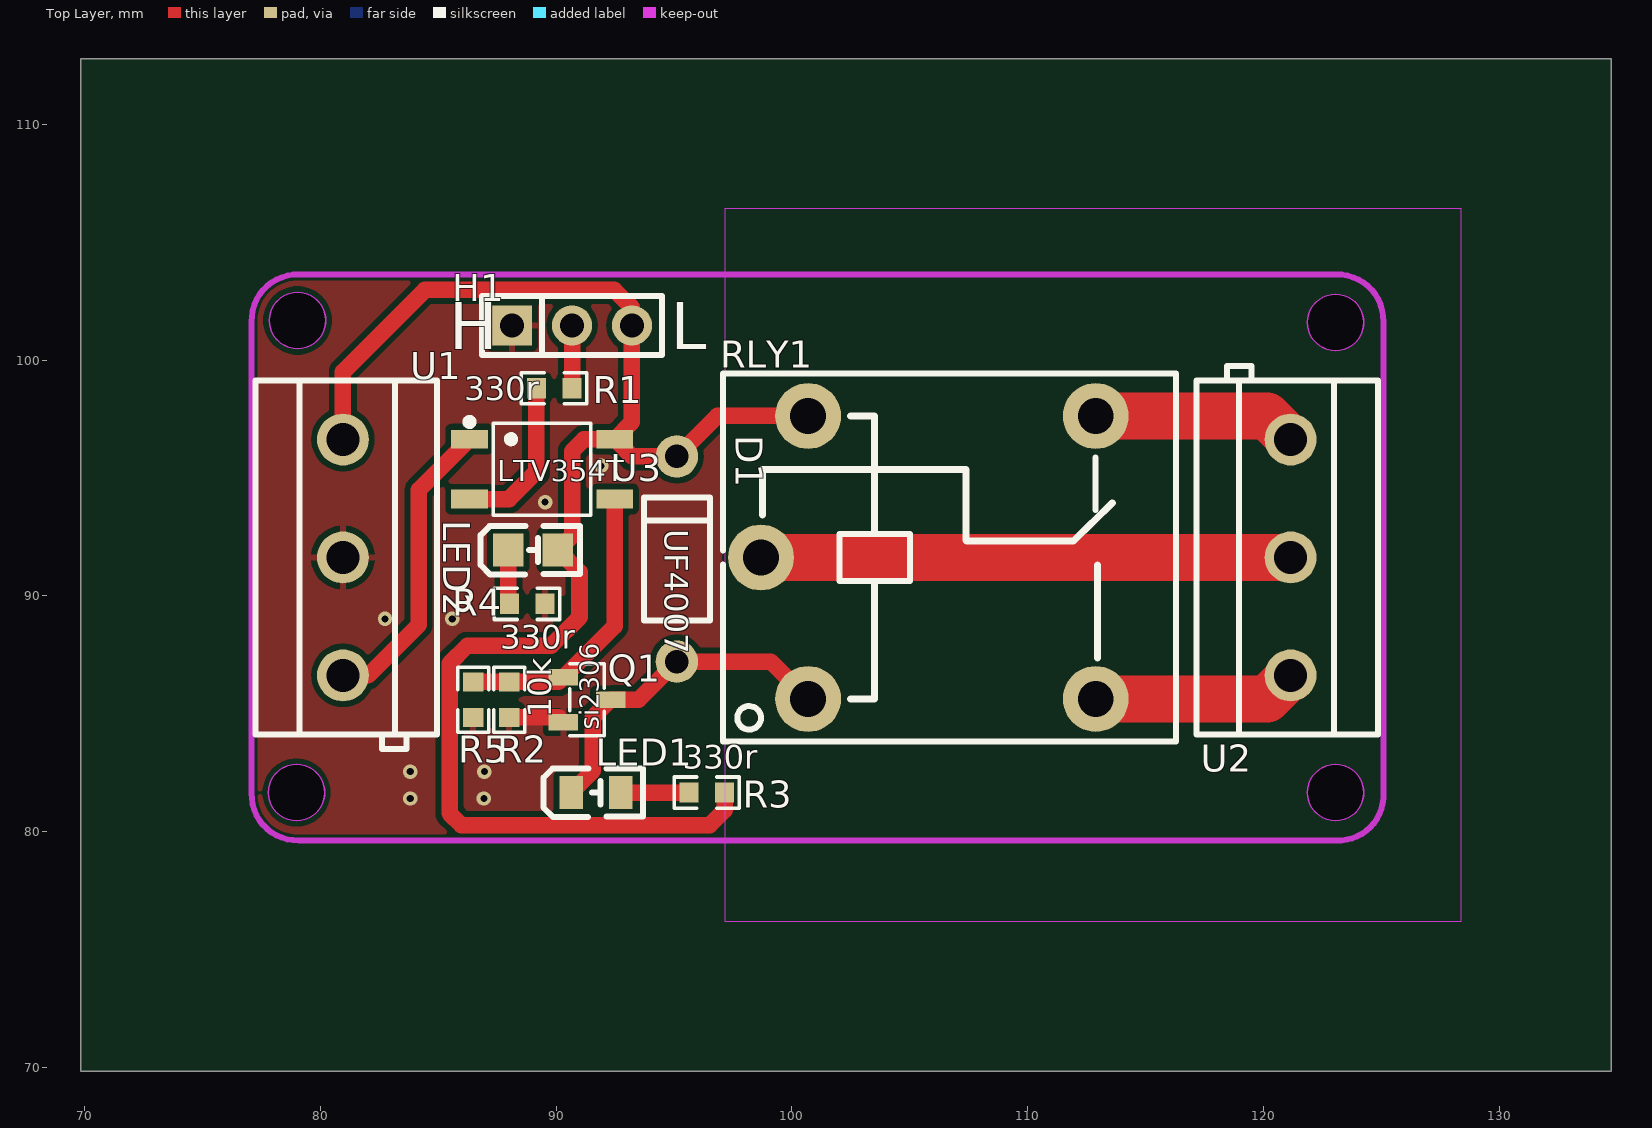
[diagram p0: Top Layer view]
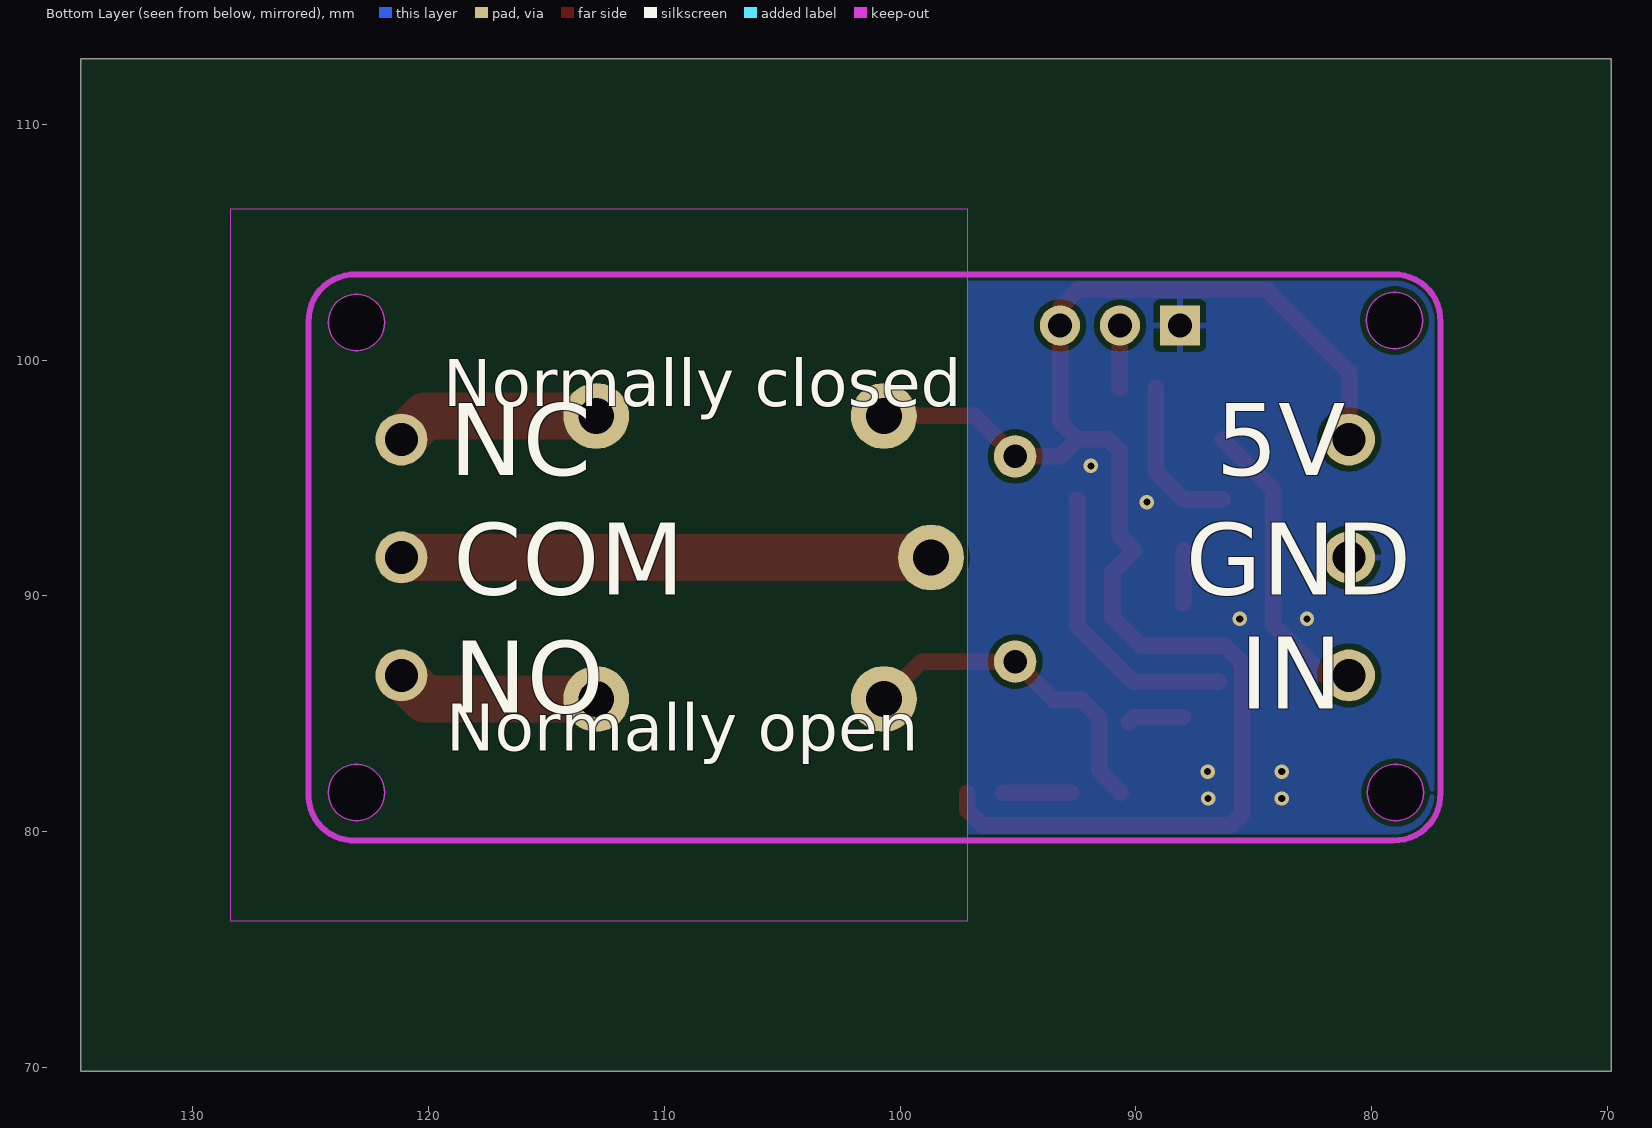
[diagram p1: Bottom Layer view, seen from below]
# Altium PCB MISC49931.pcbdoc
Units mm, origin at the board's own origin, x right, y up, seen from the top; angles counter-clockwise.
Board outline 64.9 x 42.93 mm, 2 copper layers (Top Layer, Bottom Layer), stack 1.58 mm thick; 14 components, 12 nets, 37 pads, 8 vias.

## Layer stack, top to bottom
Top Solder Mask Layer: solder mask 0.01, Dk 3.3
Top Layer: signal copper 0.035
Dielectric1: surface 1.51, FR4, Dk 4.5
Bottom Layer: signal copper 0.035
Bottom Solder Mask Layer: solder mask 0.01, Dk 3.3

## Board outline
134.747,69.85 69.85,69.85 69.85,112.776 134.747,112.776
cut-out: 80.233,101.684 cw(c79.037,101.684) 77.84,101.684 cw(c79.037,101.684)
cut-out: 80.191,81.661 cw(c78.994,81.661) 77.797,81.661 cw(c78.994,81.661)
cut-out: 124.26,81.661 cw(c123.063,81.661) 121.866,81.661 cw(c123.063,81.661)
cut-out: 124.26,101.6 cw(c123.063,101.6) 121.866,101.6 cw(c123.063,101.6)

## Design rules (kind name [scope] priority, off if disabled: settings)
BoardOutlineClearance copperThickness2oz_1 [All] p2 off: genericclearance=0.203 ignorepadtopadclearanceinfootprint=FALSE except(0: Arc-SplitContinuation Track-SplitContinuation SMDPad-SplitContinuation THPad-SplitContinuation Via-SplitContinuation Fill-SplitContinuation Region-SplitContinuation Poly-SplitContinuation Text-SplitContinuation Hole-SplitContinuation; 0.152: Arc-CutoutEdge SMDPad-CutoutEdge THPad-CutoutEdge Via-CutoutEdge Fill-CutoutEdge Region-CutoutEdge Text-CutoutEdge; 0.176: Hole-OutlineEdge Hole-CutoutEdge; 0.254: Poly-OutlineEdge Poly-CutoutEdge; 0.3: Arc-OutlineEdge Track-OutlineEdge SMDPad-OutlineEdge THPad-OutlineEdge Via-OutlineEdge Fill-OutlineEdge Region-OutlineEdge Text-OutlineEdge Track-CutoutEdge)
BoardOutlineClearance copperThickness1oz_1 [All] p4: genericclearance=0.102 ignorepadtopadclearanceinfootprint=FALSE except(0: Arc-SplitContinuation Track-SplitContinuation SMDPad-SplitContinuation THPad-SplitContinuation Via-SplitContinuation Fill-SplitContinuation Region-SplitContinuation Poly-SplitContinuation Text-SplitContinuation Hole-SplitContinuation; 0.152: SMDPad-CutoutEdge THPad-CutoutEdge Via-CutoutEdge Fill-CutoutEdge Region-CutoutEdge Text-CutoutEdge; 0.176: Hole-OutlineEdge Hole-CutoutEdge; 0.254: Poly-OutlineEdge Poly-CutoutEdge; 0.3: Arc-OutlineEdge Track-OutlineEdge SMDPad-OutlineEdge THPad-OutlineEdge Via-OutlineEdge Fill-OutlineEdge Region-OutlineEdge Text-OutlineEdge Arc-CutoutEdge Track-CutoutEdge)
Clearance copperThickness2oz [All] p1 off: gap=0.203 ignorepadtopadclearanceinfootprint=FALSE except(0.152: SMDPad-Track SMDPad-SMDPad THPad-Track SMDPad-THPad THPad-THPad Track-Via SMDPad-Via THPad-Via Via-Via Fill-Track Region-Track Fill-SMDPad Region-SMDPad Fill-THPad Region-THPad Fill-Via Region-Via Fill-Fill Fill-Region Region-Region Arc-Track Arc-SMDPad Arc-THPad Arc-Via Fill-Arc Region-Arc Arc-Arc Text-Track SMDPad-Text Text-THPad Text-Via Fill-Text Region-Text Arc-Text Text-Text; 0.176: Hole-Track Hole-SMDPad Hole-THPad Hole-Via Fill-Hole Region-Hole Hole-Arc Hole-Text; 0.254: Poly-Track Poly-SMDPad Poly-THPad Poly-Via Poly-Fill Poly-Region Poly-Poly Poly-Arc Poly-Text Poly-Hole)
Clearance copperThickness1oz [All] p3: gap=0.102 ignorepadtopadclearanceinfootprint=FALSE except(0.152: SMDPad-Track SMDPad-SMDPad THPad-Track SMDPad-THPad THPad-THPad Track-Via SMDPad-Via THPad-Via Via-Via Fill-Track Region-Track Fill-SMDPad Region-SMDPad Fill-THPad Region-THPad Fill-Via Region-Via Fill-Fill Fill-Region Region-Region Arc-Track Arc-SMDPad Arc-THPad Arc-Via Fill-Arc Region-Arc Arc-Arc Text-Track SMDPad-Text Text-THPad Text-Via Fill-Text Region-Text Arc-Text Text-Text; 0.176: Hole-Track Hole-SMDPad Hole-THPad Hole-Via Fill-Hole Region-Hole Hole-Arc Hole-Text; 0.254: Poly-Track Poly-SMDPad Poly-THPad Poly-Via Poly-Fill Poly-Region Poly-Poly Poly-Arc Poly-Text Poly-Hole)
DiffPairsRouting differentialPair [All] p1: maxlimit=0.152 minlimit=0.152 mostfreqgap=0.152 toplayer_minwidth=0.127 toplayer_prefwidth=0.254 toplayer_maxwidth=2.54 toplayer_mingap=0.152 toplayer_prefgap=0.152 toplayer_maxgap=0.152 bottomlayer_minwidth=0.127 bottomlayer_prefwidth=0.254 bottomlayer_maxwidth=2.54 bottomlayer_mingap=0.152 bottomlayer_prefgap=0.152 bottomlayer_maxgap=0.152 maxuncoupledlength=0.254
HoleToHoleClearance otherClearance [All] p1: gap=0.3 allowstackedmicrovias=TRUE
Length netLength [All] p1: minlimit=0 maxlimit=0
MatchedLengths netLengthTolerance [All] p1: tolerance=25.4
PasteMaskExpansion pasteMaskExpansion [All] p1: expansion=0
PlaneConnect innerPlane [All] p1: planeconnectstyle=Relief reliefexpansion=0.508 reliefentries=4 reliefconductorwidth=0.254 reliefairgap=0.254
PolygonConnect copperRegion [All] p1: connectstyle=Relief reliefconductorwidth=0.254 reliefentries=4 polygonreliefangle="90 Angle" airgapwidth=0.254 via.connectstyle=Relief via.reliefconductorwidth=0.254 via.reliefentries=4 via.polygonreliefangle="90 Angle" via.airgapwidth=0.254
RoutingVias viaSize [All] p1: holewidth=0.305 width=0.61 viastyle="Through Hole" minholewidth=0.3 minwidth=0.5 maxholewidth=6.3 maxwidth=10
SolderMaskExpansion solderMaskExpansion [IsVia] p1: expansion=-25.4 istentingtop=TRUE
SolderMaskExpansion solderMaskExpansion [All] p2: expansion=0.051 istentingtop=FALSE
Width copperThickness2oz_2 [All] p1 off: maxlimit=2.54 minlimit=0.203 preferedwidth=0.254
Width copperThickness1oz_2 [All] p2: maxlimit=2.54 minlimit=0.127 preferedwidth=0.254

## Components (designator, comment, footprint, x,y, rotation, side; value= is the part's Value field where it differs from the comment)
D1 "UF4007" DO-41_BD2.4-L4.7-P8.70-D0.9-RD 95.123,91.567 r270 top
H1 "PZ254V-11-03P" HDR-TH_3P-P2.54-V-M_PZ254V-11-03P 90.678,101.473 r0 top
LED1 "GL0805UR01" LED0805-R-RD_RED 91.694,81.661 r0 top
LED2 "GL0805UG01" LED0805-FD_GL0805UG01 89.027,91.948 r180 top
Q1 "SI2308A" SOT-23-3_L2.9-W1.3-P1.90-LS2.4-BR 91.313,85.598 r180 top
R1 "330Ω" R0603 89.916,98.806 r180 top
R2 "10kΩ" R0603 88.011,85.598 r90 top
R3 "330Ω" R0603 96.393,81.661 r180 top
R4 "330Ω" R0603 88.773,89.662 r0 top
R5 "10kΩ" R0603 86.487,85.598 r270 top
RLY1 "SRD-05VDC-SL-C" RELAY-TH_SRD-XXVDC-XL-C 105.791,91.632 r0 top
U1 "KF301-5.0-3P" CONN-TH_3P-P5.00_KF301-5.0-3P 80.962,91.632 r270 top
U2 "KF301-5.0-3P" CONN-TH_3P-P5.00_KF301-5.0-3P 121.158,91.632 r90 top
U3 "LTV-354T-A" SOP-4_L3.9-W4.4-P2.54-LS7.0-TL 89.408,95.377 r0 top

## Footprints (in the part's own frame and the unit in brackets; to place one, negate y for a bottom-side part, rotate by r counter-clockwise, add the part's x,y. Pads: shape width x height; smd on the part's side, far side on the other; paste and mask are expansions set on the pad)
CONN-TH_3P-P5.00_KF301-5.0-3P [mm]
  round 2.2 hole 1.4: 1(-5,0) 2(0,0) 3(5,0)
  silkscreen extent -7.5,-3.7 8.13,4
DO-41_BD2.4-L4.7-P8.70-D0.9-RD [mm]
  round 1.8 hole 1: 1(-4.35,0) 2(4.35,0)
  silkscreen extent -2.6,-1.4 2.6,1.4
HDR-TH_3P-P2.54-V-M_PZ254V-11-03P [mm]
  rect 1.7x1.7 hole 1.02: 1(-2.54,0)
  round 1.7 hole 1.02: 2(0,0) 3(2.54,0)
  silkscreen extent -3.81,-1.25 3.81,1.25
LED0805-FD_GL0805UG01 [mm]
  rect 1.3x1.4 smd: 1(-1.05,0) 2(1.05,0)
  silkscreen extent -1.99,-1.01 2.22,1.04
LED0805-R-RD_RED [mm]
  rect 1x1.4 smd: 1(1.05,0) 2(-1.05,0)
  silkscreen extent -2.22,-1.04 1.99,1.01
R0603 [mm]
  rect 0.806x0.864 smd paste-100 mask+0.051: 1(-0.753,0) 2(0.753,0)
  silkscreen extent -1.39,-0.66 1.39,0.66
RELAY-TH_SRD-XXVDC-XL-C [mil]
  round 110 hole 60: 1(-200.79,-236.22) 2(279.52,-236.2) 3(279.53,236.2) 4(-200.79,236.22) 5(-279.53,0)
  silkscreen extent -342,-307 413,307
SOP-4_L3.9-W4.4-P2.54-LS7.0-TL [mm]
  rect 1.56x0.8 smd: 1(-3.08,1.27) 2(-3.08,-1.27) 3(3.08,-1.27) 4(3.08,1.27)
  silkscreen extent -3.23,-1.95 2.07,2.15
SOT-23-3_L2.9-W1.3-P1.90-LS2.4-BR [mm]
  rect 1.25x0.7 smd: 1(1,-0.95) 2(1,0.95) 3(-1,0)
  silkscreen extent -0.73,-1.53 0.73,1.53

## Via types
v1: diameter 0.61, hole 0.305, Top Layer to Bottom Layer, 8 vias

## Nets (pads, with @x,y where several pads share a name; then routed paths per layer and width w, separated by ;. In a path a pad name is that pad's centre, name@x,y a point inside that pad or via, vN(x,y) a via of type N, cw(c..) or ccw(c..) an arc to the next point about the centre after c; other vN are vias at no path point)
$1N1: LED2.2 R4.1 | length 2.3
  Top Layer w0.7: LED2.2 87.977,89.705 R4.1
$1N2: LED1.1 R3.2 | length 2.9
  Top Layer w0.7: LED1.1@92.744,81.661 R3.2
$1N6: H1.2 R1.1 | length 2.7
  Top Layer w0.7: R1.1 90.678,98.815 H1.2
$1N7: R1.2 U3.2 | length 6.9
  Top Layer w0.7: U3.2 88.011,94.107 89.154,95.25 89.154,98.797 R1.2
$1N15: D1.2 LED1.2 Q1.3 RLY1.1 | length 14.3
  Top Layer w0.7: LED1.2@90.644,81.661 91.567,82.584 91.567,84.852 Q1.3 93.504,85.598 D1.2 99.106,87.217 RLY1.1
$1N22: Q1.1 R2.2 R5.1 U3.3 | length 12.4
  Top Layer w0.7: R5.1 R2.2 90.116,86.351 Q1.1 92.488,88.723 U3.3
+5V: D1.1 H1.3 LED2.1 R3.1 RLY1.4 U1.1 U3.4 | length 67.2
  Top Layer w0.7: U1.1 80.962,99.504 84.44,102.982 92.471,102.982 93.218,102.235 H1.3 93.218,97.377 U3.4 ; R3.1 97.146,80.908 96.52,80.282 85.979,80.282 85.484,80.777 85.484,87.135 86.233,87.884 89.789,87.884 90.995,89.09 90.995,91.03 LED2.1 90.678,92.549 90.678,96.139 91.186,96.647 U3.4 ; RLY1.4 96.838,97.632 D1.1 93.218,95.917 U3.4
COM: RLY1.5 U2.2 | length 22.5
  Top Layer w2: RLY1.5 U2.2
GND: H1.1 Q1.2 R2.1 R4.2 R5.2 U1.2 | length 2.4
  Top Layer w0.7: R2.1 90.116,84.845 Q1.2
  other v1: 83.82,81.407 86.939,81.407 83.82,82.55 86.962,82.55 82.747,89.027 85.598,89.027 89.535,93.98 91.912,95.514
IN: U1.3 U3.1 | length 12.9
  Top Layer w0.7: U1.3 82.034,86.632 84.175,88.773 84.175,94.494 U3.1
NC: RLY1.3 U2.3 | length 8.7
  Top Layer w2: RLY1.3 120.159,97.631 U2.3
NO: RLY1.2 U2.1 | length 8.7
  Top Layer w2: RLY1.2 120.159,85.633 U2.1

## Polygon pours and split planes (outlines as drawn)
GND on Top Layer (solid, remove dead copper, pour order 0): 77.089,103.632 77.089,79.248 125.603,79.248 125.603,103.632
GND on Bottom Layer (solid, remove dead copper, pour order 2): 76.2,104.394 76.2,78.105 126.619,78.105 126.619,104.394

## Keep-outs
Board Outline Layer:
  region: 97.155,106.426 97.155,76.2 128.397,76.2 128.397,106.426
  region: 80.233,101.684 cw(c79.037,101.684) 77.84,101.684 cw(c79.037,101.684)
  circle w0.003: c79.037,101.684 r1.197
  region: 80.233,101.684 80.224,101.534 80.196,101.387 80.149,101.244 80.085,101.108 80.005,100.981 79.909,100.865 79.8,100.762 79.678,100.674 79.546,100.601 79.407,100.546 79.261,100.509 79.112,100.49 78.962,100.49 78.813,100.509 78.667,100.546 78.527,100.601 78.396,100.674 78.274,100.762 78.165,100.865 78.069,100.981 77.988,101.108 77.924,101.244 77.878,101.387 77.85,101.534 77.84,101.684 77.85,101.834 77.878,101.982 77.924,102.125 77.988,102.261 78.069,102.387 78.165,102.503 78.274,102.606 78.396,102.694 78.527,102.767 78.667,102.822 78.813,102.859 78.962,102.878 79.112,102.878 79.261,102.859 79.407,102.822 79.546,102.767 79.678,102.694 79.8,102.606 79.909,102.503 80.005,102.387 80.085,102.261 80.149,102.125 80.196,101.982 80.224,101.834
  region: 80.191,81.661 cw(c78.994,81.661) 77.797,81.661 cw(c78.994,81.661)
  circle w0.003: c78.994,81.661 r1.197
  region: 80.191,81.661 80.181,81.511 80.153,81.363 80.107,81.221 80.043,81.085 79.962,80.958 79.866,80.842 79.757,80.739 79.635,80.651 79.503,80.578 79.364,80.523 79.218,80.486 79.069,80.467 78.919,80.467 78.77,80.486 78.624,80.523 78.485,80.578 78.353,80.651 78.231,80.739 78.122,80.842 78.026,80.958 77.945,81.085 77.881,81.221 77.835,81.363 77.807,81.511 77.797,81.661 77.807,81.811 77.835,81.959 77.881,82.101 77.945,82.237 78.026,82.364 78.122,82.48 78.231,82.583 78.353,82.671 78.485,82.744 78.624,82.799 78.77,82.836 78.919,82.855 79.069,82.855 79.218,82.836 79.364,82.799 79.503,82.744 79.635,82.671 79.757,82.583 79.866,82.48 79.962,82.364 80.043,82.237 80.107,82.101 80.153,81.959 80.181,81.811
  region: 124.26,81.661 cw(c123.063,81.661) 121.866,81.661 cw(c123.063,81.661)
  circle w0.003: c123.063,81.661 r1.197
  region: 124.26,81.661 124.25,81.511 124.222,81.363 124.176,81.221 124.112,81.085 124.031,80.958 123.935,80.842 123.826,80.739 123.704,80.651 123.572,80.578 123.433,80.523 123.287,80.486 123.138,80.467 122.988,80.467 122.839,80.486 122.693,80.523 122.554,80.578 122.422,80.651 122.3,80.739 122.191,80.842 122.095,80.958 122.014,81.085 121.95,81.221 121.904,81.363 121.876,81.511 121.866,81.661 121.876,81.811 121.904,81.959 121.95,82.101 122.014,82.237 122.095,82.364 122.191,82.48 122.3,82.583 122.422,82.671 122.554,82.744 122.693,82.799 122.839,82.836 122.988,82.855 123.138,82.855 123.287,82.836 123.433,82.799 123.572,82.744 123.704,82.671 123.826,82.583 123.935,82.48 124.031,82.364 124.112,82.237 124.176,82.101 124.222,81.959 124.25,81.811
  region: 124.26,101.6 cw(c123.063,101.6) 121.866,101.6 cw(c123.063,101.6)
  circle w0.003: c123.063,101.6 r1.197
  region: 124.26,101.6 124.25,101.45 124.222,101.302 124.176,101.16 124.112,101.024 124.031,100.897 123.935,100.781 123.826,100.678 123.704,100.59 123.572,100.517 123.433,100.462 123.287,100.425 123.138,100.406 122.988,100.406 122.839,100.425 122.693,100.462 122.554,100.517 122.422,100.59 122.3,100.678 122.191,100.781 122.095,100.897 122.014,101.024 121.95,101.16 121.904,101.302 121.876,101.45 121.866,101.6 121.876,101.75 121.904,101.898 121.95,102.04 122.014,102.176 122.095,102.303 122.191,102.419 122.3,102.522 122.422,102.61 122.554,102.683 122.693,102.738 122.839,102.775 122.988,102.794 123.138,102.794 123.287,102.775 123.433,102.738 123.572,102.683 123.704,102.61 123.826,102.522 123.935,102.419 124.031,102.303 124.112,102.176 124.176,102.04 124.222,101.898 124.25,101.75
  lines w0.254: 77.089,81.632 ccw(c79.037,81.58) 79.089,79.632 123.089,79.632 ccw(c123.183,81.538) 125.089,81.632 125.089,101.632 ccw(c123.141,101.684) 123.089,103.632 79.089,103.632 ccw(c79.037,101.684) 77.089,101.632 77.089,81.632

## Silkscreen, mask and mechanical layers (free items; w line width, h text height)
Top Silkscreen Layer:
  text "H" at 85.471,100.457 h2
  text "L" at 94.864,100.457 h2
  text "330r" at 86.106,98.298 h1
  text "LTV354T" at 87.503,94.869 h0.9
  text "UF4007" at 94.615,92.837 h1 r270
  text "330r" at 87.63,87.757 h1
  text "10k" at 89.789,84.836 h1 r90
  text "si2306" at 91.821,84.328 h0.8 r90
  text "330r" at 95.377,82.677 h1
Bottom Silkscreen Layer:
  text "Normally closed" at 119.38,98.044 h2
  text "5V" at 86.614,95.123 h3.05
  text "NC" at 119.126,95.123 h3.05
  text "COM" at 118.957,90.061 h3.05
  text "GND" at 87.884,90.043 h3.05
  text "IN" at 85.598,85.217 h3.05
  text "NO" at 118.957,85.044 h3.05
  text "Normally open" at 119.253,83.439 h2
Mechanical Layer:
  circle w0.003: c79.037,101.684 r1.197
  circle w0.003: c78.994,81.661 r1.197
  circle w0.003: c123.063,81.661 r1.197
  circle w0.003: c123.063,101.6 r1.197